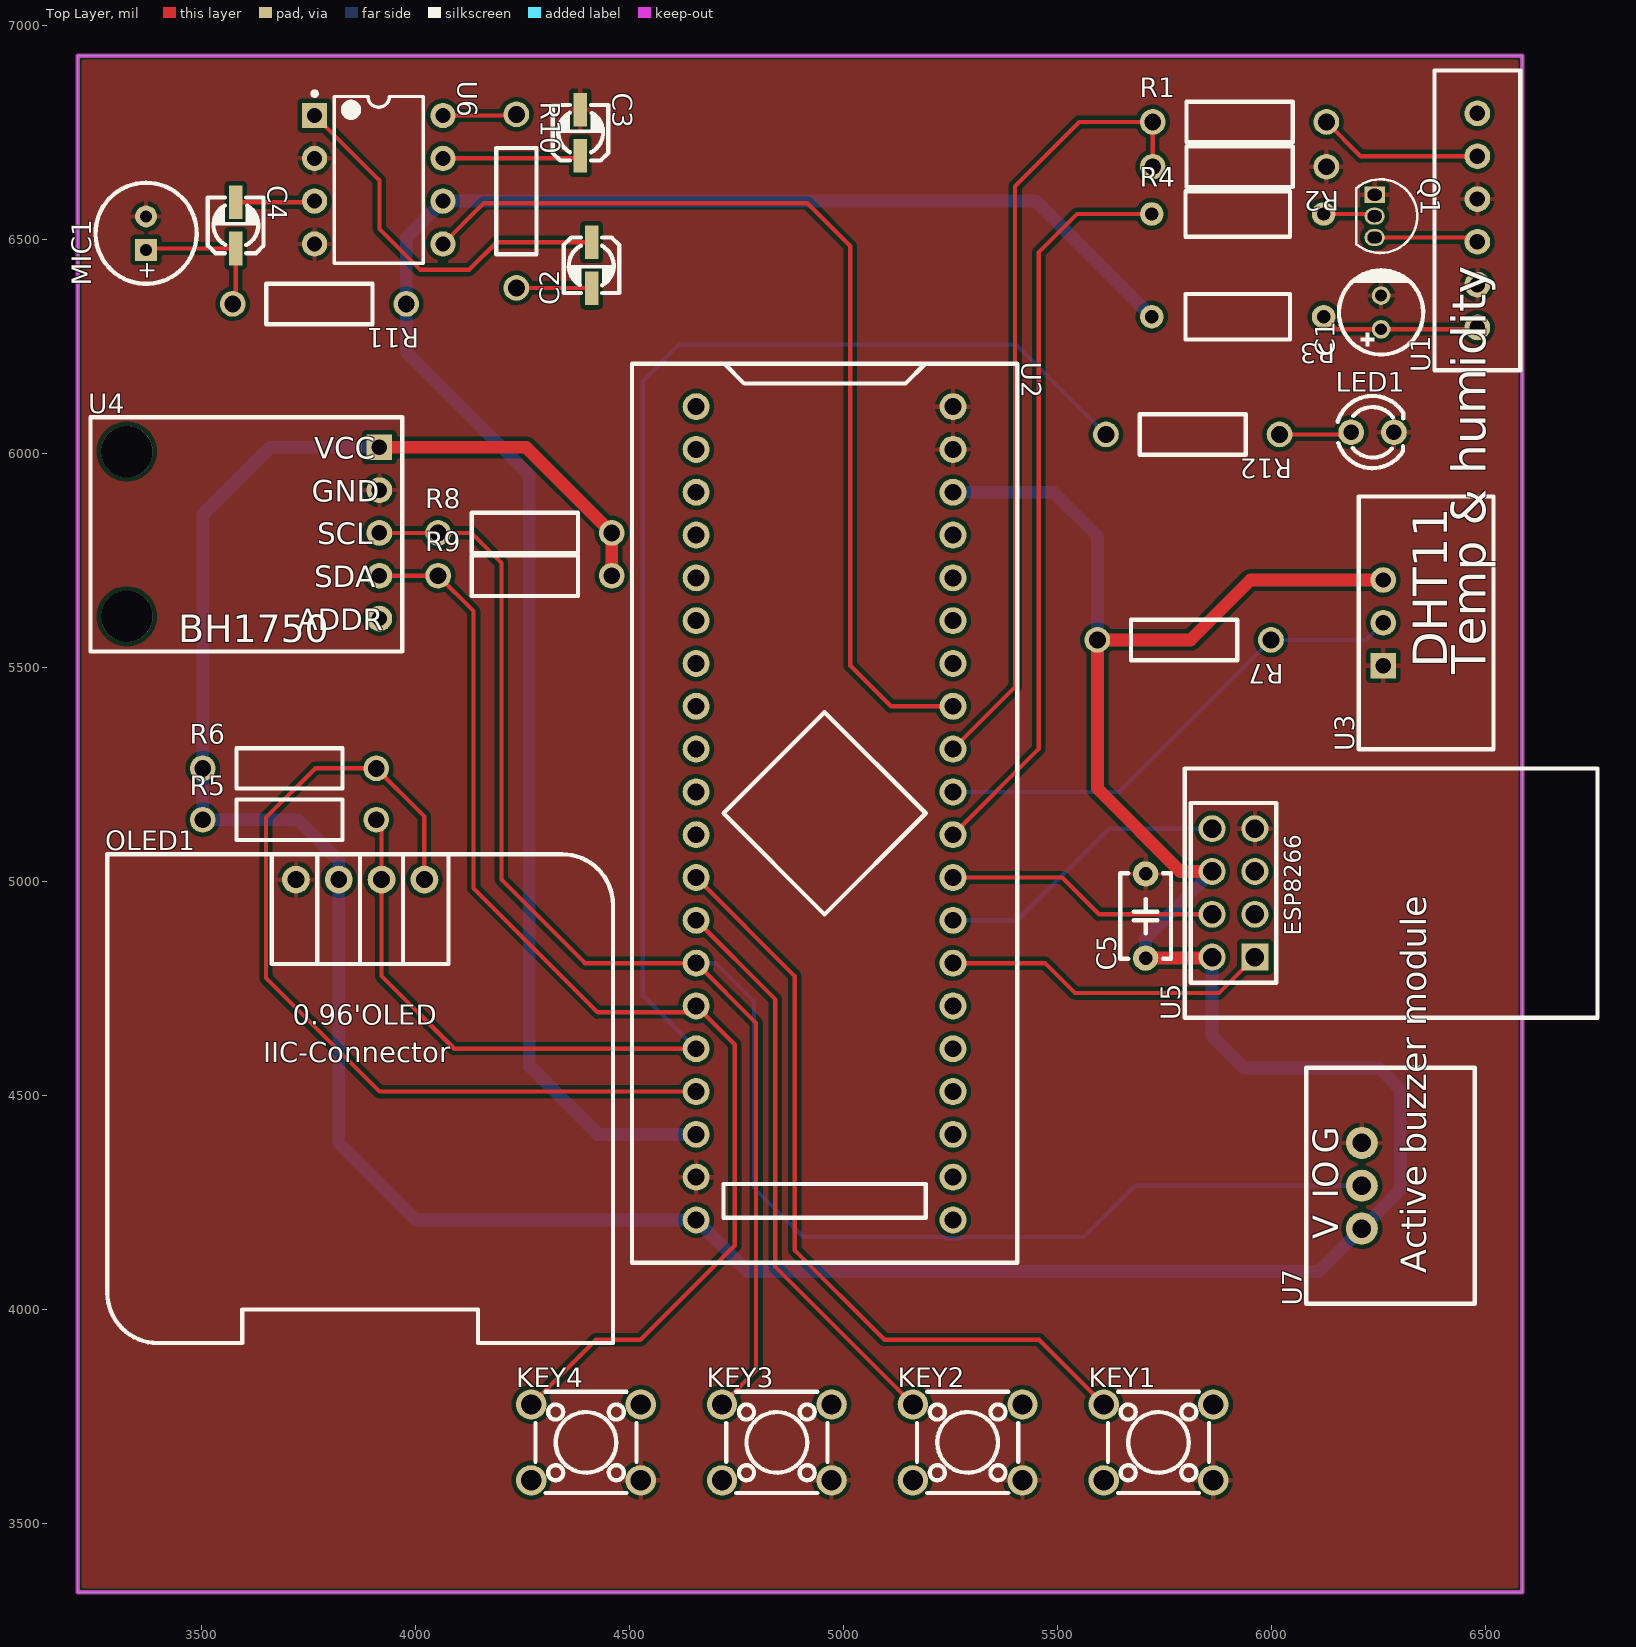
[diagram p0: Top Layer view]
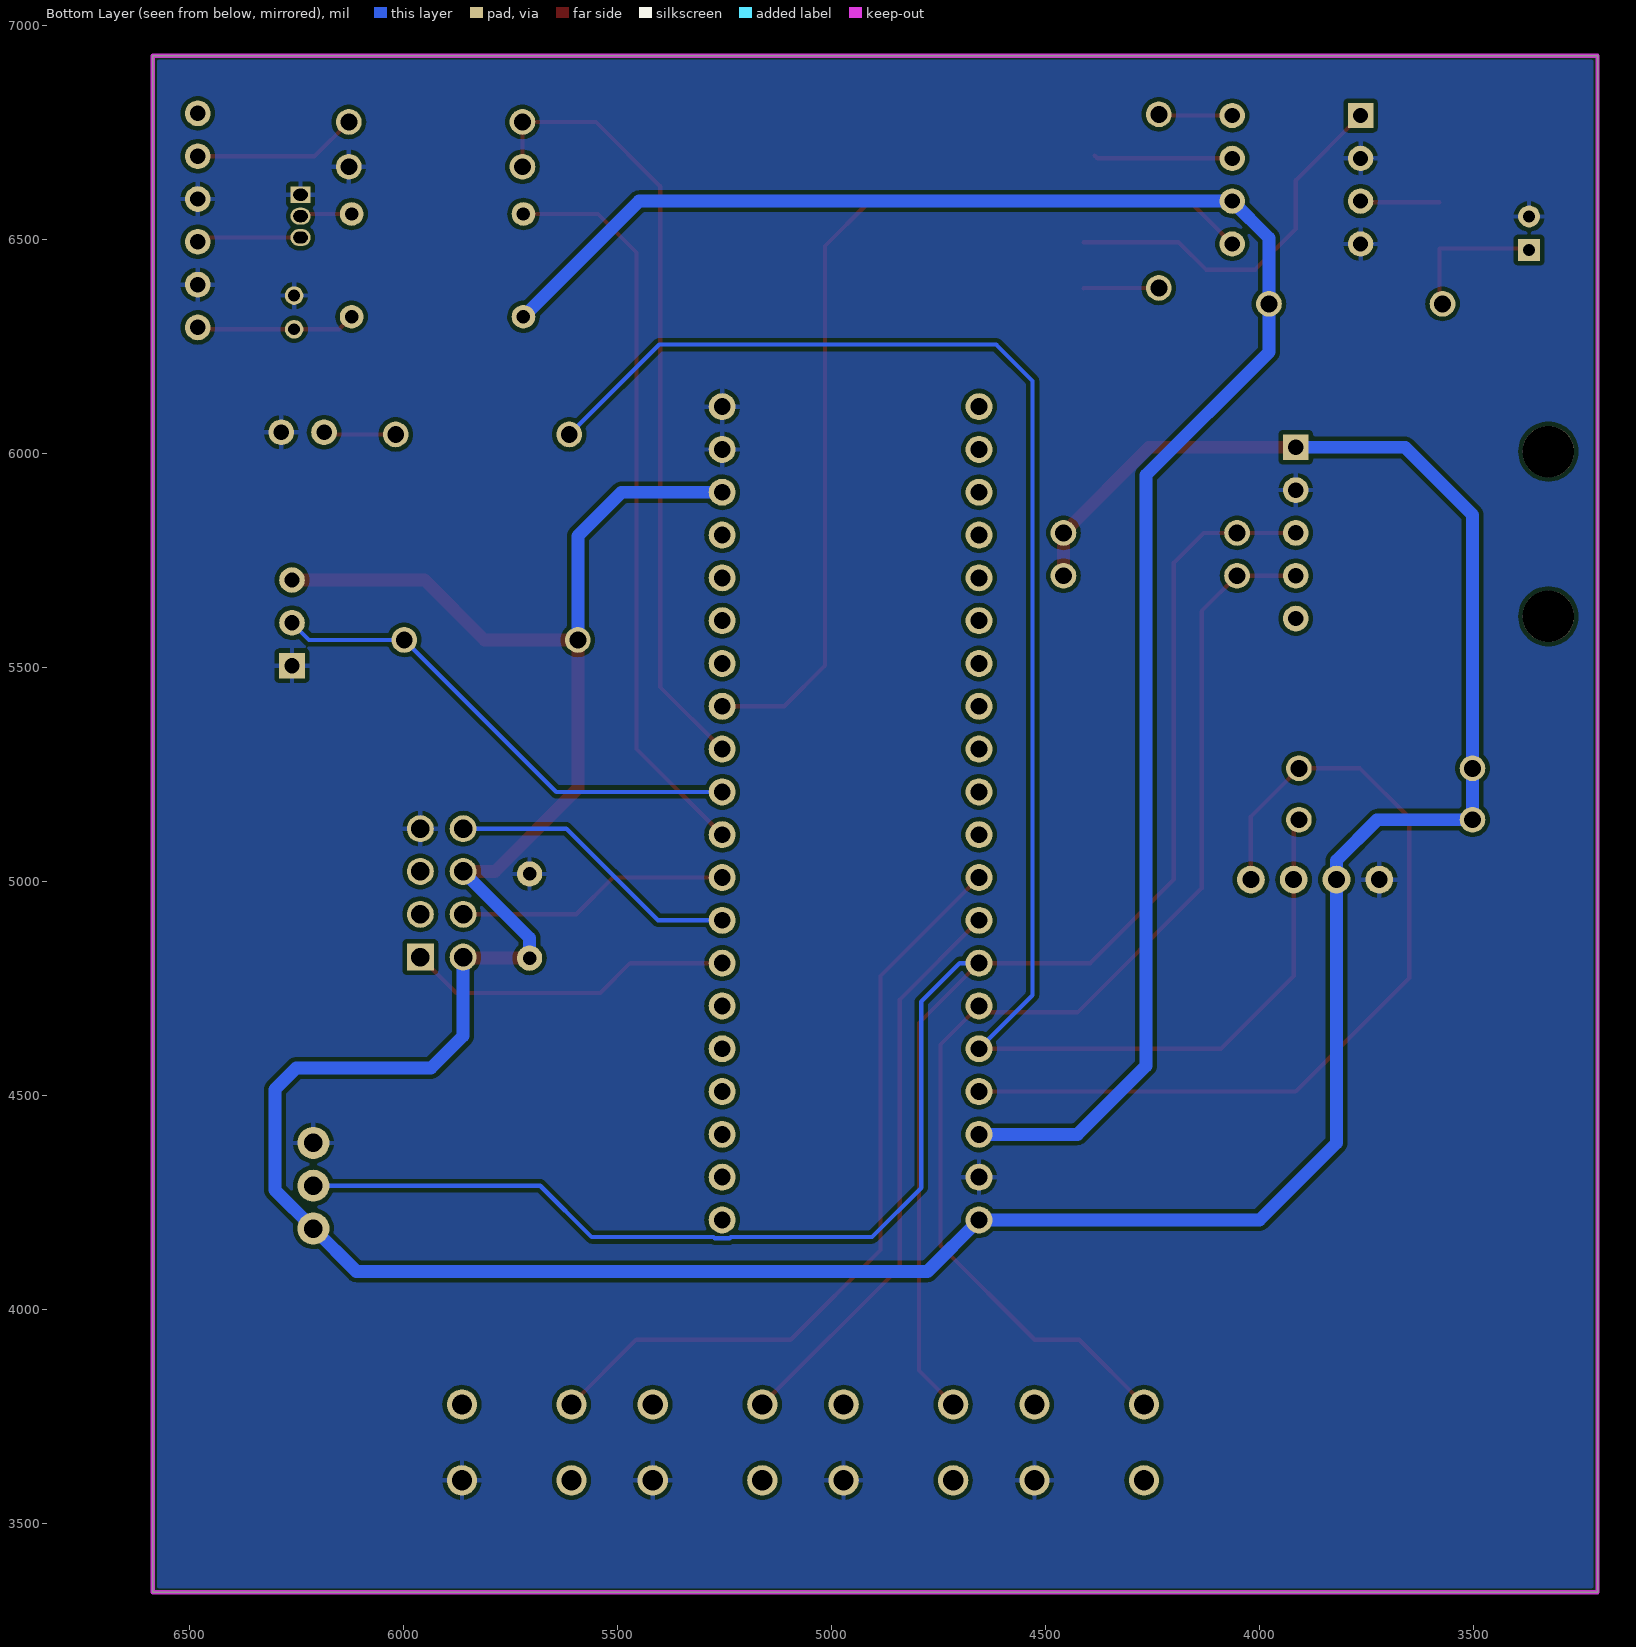
[diagram p1: Bottom Layer view, seen from below]
# Altium PCB MISC52092.pcbdoc
Units mil, origin at the board's own origin, x right, y up, seen from the top; angles counter-clockwise.
Board outline 3375 x 3590 mil, 2 copper layers (Top Layer, Bottom Layer), stack 62.206 mil thick; 32 components, 48 nets, 136 pads, 0 vias.

## Layer stack, top to bottom
Top Solder Mask Layer: solder mask 0.394, Dk 3.3
Top Layer: signal copper 1.379
Dielectric1: surface 59.449, FR4, Dk 4.5
Bottom Layer: signal copper 1.378
Bottom Solder Mask Layer: solder mask 0.394, Dk 3.3

## Board outline
3210,6930 3210,3340 6585,3340 6585,6930

## Design rules (kind name [scope] priority, off if disabled: settings)
BoardOutlineClearance copperThickness2oz_1 [All] p2 off: genericclearance=7.99 ignorepadtopadclearanceinfootprint=FALSE except(0: Arc-SplitContinuation Track-SplitContinuation SMDPad-SplitContinuation THPad-SplitContinuation Via-SplitContinuation Fill-SplitContinuation Region-SplitContinuation Poly-SplitContinuation Text-SplitContinuation Hole-SplitContinuation; 5.98: Arc-CutoutEdge SMDPad-CutoutEdge THPad-CutoutEdge Via-CutoutEdge Fill-CutoutEdge Region-CutoutEdge Text-CutoutEdge; 6.93: Hole-OutlineEdge Hole-CutoutEdge; 10: Poly-OutlineEdge Poly-CutoutEdge; 11.81: Arc-OutlineEdge Track-OutlineEdge SMDPad-OutlineEdge THPad-OutlineEdge Via-OutlineEdge Fill-OutlineEdge Region-OutlineEdge Text-OutlineEdge Track-CutoutEdge)
BoardOutlineClearance copperThickness1oz_1 [All] p4: genericclearance=4.02 ignorepadtopadclearanceinfootprint=FALSE except(0: Arc-SplitContinuation Track-SplitContinuation SMDPad-SplitContinuation THPad-SplitContinuation Via-SplitContinuation Fill-SplitContinuation Region-SplitContinuation Poly-SplitContinuation Text-SplitContinuation Hole-SplitContinuation; 6: SMDPad-CutoutEdge THPad-CutoutEdge Via-CutoutEdge Fill-CutoutEdge Region-CutoutEdge Text-CutoutEdge; 6.93: Hole-OutlineEdge Hole-CutoutEdge; 10: Poly-OutlineEdge Poly-CutoutEdge; 11.8: Arc-OutlineEdge Track-OutlineEdge SMDPad-OutlineEdge THPad-OutlineEdge Via-OutlineEdge Fill-OutlineEdge Region-OutlineEdge Text-OutlineEdge; 11.81: Arc-CutoutEdge Track-CutoutEdge)
Clearance copperThickness2oz [All] p1 off: gap=7.99 ignorepadtopadclearanceinfootprint=FALSE except(5.98: SMDPad-Track SMDPad-SMDPad THPad-Track SMDPad-THPad THPad-THPad Track-Via SMDPad-Via THPad-Via Via-Via Fill-Track Region-Track Fill-SMDPad Region-SMDPad Fill-THPad Region-THPad Fill-Via Region-Via Fill-Fill Fill-Region Region-Region Arc-Track Arc-SMDPad Arc-THPad Arc-Via Fill-Arc Region-Arc Arc-Arc Text-Track SMDPad-Text Text-THPad Text-Via Fill-Text Region-Text Arc-Text Text-Text; 6.93: Hole-Track Hole-SMDPad Hole-THPad Hole-Via Fill-Hole Region-Hole Hole-Arc Hole-Text; 10: Poly-Track Poly-SMDPad Poly-THPad Poly-Via Poly-Fill Poly-Region Poly-Poly Poly-Arc Poly-Text Poly-Hole)
Clearance copperThickness1oz [All] p3: gap=4.02 ignorepadtopadclearanceinfootprint=FALSE except(5.98: SMDPad-Track SMDPad-SMDPad THPad-Track SMDPad-THPad THPad-THPad Track-Via SMDPad-Via THPad-Via Via-Via Fill-Track Region-Track Fill-SMDPad Region-SMDPad Fill-THPad Region-THPad Fill-Via Region-Via Fill-Fill Fill-Region Region-Region; 6: Arc-Track Arc-SMDPad Arc-THPad Arc-Via Fill-Arc Region-Arc Arc-Arc Text-Track SMDPad-Text Text-THPad Text-Via Fill-Text Region-Text Arc-Text Text-Text; 6.93: Hole-Track Hole-SMDPad Hole-THPad Hole-Via Fill-Hole Region-Hole Hole-Arc Hole-Text; 10: Poly-Track Poly-SMDPad Poly-THPad Poly-Via Poly-Fill Poly-Region Poly-Poly Poly-Arc Poly-Text Poly-Hole)
DiffPairsRouting differentialPair [All] p1: maxlimit=6 minlimit=6 mostfreqgap=6 toplayer_minwidth=5 toplayer_prefwidth=10 toplayer_maxwidth=100 toplayer_mingap=6 toplayer_prefgap=6 toplayer_maxgap=6 bottomlayer_minwidth=5 bottomlayer_prefwidth=10 bottomlayer_maxwidth=100 bottomlayer_mingap=6 bottomlayer_prefgap=6 bottomlayer_maxgap=6 maxuncoupledlength=10
HoleToHoleClearance otherClearance [All] p1: gap=11.81 allowstackedmicrovias=TRUE
Length netLength [All] p1: minlimit=0 maxlimit=0
MatchedLengths netLengthTolerance [All] p1: tolerance=1000
PasteMaskExpansion pasteMaskExpansion [All] p1: expansion=0
PlaneConnect innerPlane [All] p1: planeconnectstyle=Relief reliefexpansion=20 reliefentries=4 reliefconductorwidth=10 reliefairgap=10
PolygonConnect copperRegion [(InNet('GND'))] p1: connectstyle=Relief reliefconductorwidth=10 reliefentries=4 polygonreliefangle="90 Angle" airgapwidth=10 via.connectstyle=Relief via.reliefconductorwidth=10 via.reliefentries=4 via.polygonreliefangle="90 Angle" via.airgapwidth=10
RoutingVias viaSize [All] p1: holewidth=12.01 width=24.02 viastyle="Through Hole" minholewidth=11.81 minwidth=19.68 maxholewidth=248.03 maxwidth=393.7
SolderMaskExpansion solderMaskExpansion [IsVia] p1: expansion=-1000 istentingtop=TRUE
SolderMaskExpansion solderMaskExpansion [All] p2: expansion=2 istentingtop=FALSE
Width copperThickness2oz_2 [All] p1 off: maxlimit=100 minlimit=8 preferedwidth=10
Width copperThickness1oz_2 [All] p2: maxlimit=100 minlimit=5 preferedwidth=10

## Components (designator, comment, footprint, x,y, rotation, side; value= is the part's Value field where it differs from the comment)
C1 "10uF" CAP-TH_BD5.0-P2.00-D0.5-FD 6255,6330 r90 top
C2 "10uF" C_Ele_SMD_3x5.4mm 4410,6440 r90 top
C3 "10uF" C_Ele_SMD_3x5.4mm 4385,6750 r270 top
C4 "10uF" C_Ele_SMD_3x5.4mm 3579.65,6533.55 r270 top
C5 "5pF" CAP-TH_L5.0-W3.0-P5.00-D0.6 5705,4920 r90 top
KEY1 "" SW-TH_4P-L6.0-W6.0-P4.50-LS6.5 5735,3690.4 r0 top
KEY2 "" SW-TH_4P-L6.0-W6.0-P4.50-LS6.5 5289.21,3690.4 r0 top
KEY3 "" SW-TH_4P-L6.0-W6.0-P4.50-LS6.5 4843.42,3690.4 r0 top
KEY4 "" SW-TH_4P-L6.0-W6.0-P4.50-LS6.5 4397.63,3690.4 r0 top
LED1 "" LED_TH-3mm 6235,6050 r0 top
MIC1 "MIC" MIC-TH_BD6.0-P2.00 3370,6515 r90 top
OLED1 "0.96OLED_4P_MODULE_JX" 0.96OLED_4P 3870,5005 r0 top
Q1 "S8050" TO-92-3_L4.5-W3.5-P1.27-L 6240,6555 r270 top
R1 "10kΩ" Res_1/4W 5924.41,6775 r0 top
R2 "10kΩ" Res_1/4W 5924.41,6670.45 r180 top
R3 "10kΩ" RES-TH_BD2.7-L6.2-P10.20-D0.4 5920,6320 r180 top
R4 "1kΩ" RES-TH_BD2.7-L6.2-P10.20-D0.4 5920,6560 r0 top
R5 "10kΩ" Res_1/4W 3705,5145 r0 top
R6 "10kΩ" Res_1/4W 3705,5265 r0 top
R7 "4.7K" Res_1/4W 5795,5565 r180 top
R8 "10kΩ" Res_1/4W 4255,5815 r0 top
R9 "10kΩ" Res_1/4W 4255,5715 r0 top
R10 "3kΩ" Res_1/4W 4235,6590 r270 top
R11 "100kΩ" Res_1/4W 3775,6350 r180 top
R12 "10kΩ" Res_1/4W 5815,6045 r180 top
U1 "PM2.5 sensor_GP2Y1014AU" PM2.5传感器_GP2Y1014AU 6480,6295 r90 top
U2 "STM32F103C8T6-Card" CONN-TH_L53.3-W22.9_STM32F103C8T6-CARD 4955,5160 r270 top
U3 "DHT11" DHT11 6460,5505 r90 top
U4 "" BH1750光照传感器 3655,5805 r0 top
U5 "" ESP8266-1 5910.21,4974.09 r90 top
U6 "LM386N-3/NOPB" DIP-8_L9.8-W6.6-P2.54-LS7.6-BL 3913.53,6640 r270 top
U7 "" 有源蜂鸣器模块 6210,4190 r90 top

## Footprints (in the part's own frame and the unit in brackets; to place one, negate y for a bottom-side part, rotate by r counter-clockwise, add the part's x,y. Pads: shape width x height; smd on the part's side, far side on the other; paste and mask are expansions set on the pad)
0.96OLED_4P [mm]
  round 1.65 hole 1 copper offset 0,0: 1(-3.81,-0.001) 2(-1.27,0.002) 3(1.27,0.002) 4(3.81,0.002)
  silkscreen extent -15,-27.5 15,1.5
BH1750光照传感器 [mil]
  rect 60x60 hole 36: 1(260,210)
  round 60 hole 36: 2(260,110) 3(260,10) 4(260,-90) 5(260,-190)
  round 120 hole 120 unplated: ""(-330,-185) ""(-330,200)
  silkscreen extent -415,-267 313,280
C_Ele_SMD_3x5.4mm [mil]
  rect 78.7x31.5 smd paste+0 mask+2: 1(54.1,-0.55) 2(-53.7,-0.55)
  silkscreen extent -65,-65 65,65
CAP-TH_BD5.0-P2.00-D0.5-FD [mm]
  round 1.1 hole 0.7 paste+0 mask+0.05: 1(-1,0) 2(1,0)
  silkscreen extent -2.5,-2.5 2.5,2.5
CAP-TH_L5.0-W3.0-P5.00-D0.6 [mm]
  round 1.5 hole 0.8: 1(-2.5,0) 2(2.5,0)
  silkscreen extent -2.54,-1.5 2.54,1.5
CONN-TH_L53.3-W22.9_STM32F103C8T6-CARD [mm]
  round 1.6 hole 1: 1(-24.13,-7.62) 2(-21.59,-7.62) 3(-19.05,-7.62) 4(-16.51,-7.62) 5(-13.97,-7.62) 6(-11.43,-7.62) 7(-8.89,-7.62) 8(-6.35,-7.62) 9(-3.81,-7.62) 10(-1.27,-7.62) 11(1.27,-7.62) 12(3.81,-7.62) 13(6.35,-7.62) 14(8.89,-7.62) 15(11.43,-7.62) 16(13.97,-7.62) 17(16.51,-7.62) 18(19.05,-7.62) 19(21.59,-7.62) 20(24.13,-7.62) 21(24.13,7.62) 22(21.59,7.62) 23(19.05,7.62) 24(16.51,7.62) 25(13.97,7.62) 26(11.43,7.62) 27(8.89,7.62) 28(6.35,7.62) 29(3.81,7.62) 30(1.27,7.62) 31(-1.27,7.62) 32(-3.81,7.62) 33(-6.35,7.62) 34(-8.89,7.62) 35(-11.43,7.62) 36(-13.97,7.62) 37(-16.51,7.62) 38(-19.05,7.62) 39(-21.59,7.62) 40(-24.13,7.62)
  silkscreen extent -26.67,-11.43 26.67,11.43
DHT11 [mil]
  rect 60x60 hole 36 paste+0 mask+4: 1(-0.01,200.01)
  round 60 hole 36 paste+0 mask+2: 2(99.99,200.01)
  round 60 hole 36 paste+0 mask+4: 3(199.99,200.01)
  silkscreen extent -195,-57 395,257
DIP-8_L9.8-W6.6-P2.54-LS7.6-BL [mm]
  rect 1.5x1.5 hole 0.9: 1(-3.81,-3.81)
  round 1.5 hole 0.9: 2(-1.27,-3.81) 3(1.27,-3.81) 4(3.81,-3.81) 5(3.81,3.81) 6(1.27,3.81) 7(-1.27,3.81) 8(-3.81,3.81)
  silkscreen extent -5.23,-3.93 4.96,2.65
ESP8266-1 [mm]
  rect 1.6x1.6 hole 1.1: 1(-3.81,-1.27)
  round 1.6 hole 1.1: 2(-3.81,1.27) 3(-1.27,-1.27) 4(-1.27,1.27) 5(1.27,-1.27) 6(1.27,1.27) 7(3.81,-1.27) 8(3.81,1.27)
  silkscreen extent -7.42,-21.6 7.38,2.9
LED_TH-3mm [mil]
  round 60 hole 36 paste+0 mask+2: 1(-50,0) 2(50,0)
  silkscreen extent -81,-84 72,85
MIC-TH_BD6.0-P2.00 [mm]
  rect 1.3x1.3 hole 0.7: 1(-1,0)
  round 1.3 hole 0.7: 2(1,0)
  silkscreen extent -3,-3 3,3
PM2.5传感器_GP2Y1014AU [mil]
  round 60 hole 36 paste+0 mask+4: 1(0,0) 2(100,0) 3(200,0) 4(300,0) 5(400,0) 6(500,0)
  silkscreen extent -100,-100 600,100
RES-TH_BD2.7-L6.2-P10.20-D0.4 [mm]
  round 1.4 hole 0.8 copper offset 0,0: 1(-5.1,0) 2(5.1,0)
  silkscreen extent -3.1,-1.35 3.1,1.35
Res_1/4W [mil]
  round 60 hole 39.37 paste+0 mask+2: 1(-202.76,0) 2(202.76,0)
  silkscreen extent -124,-47 124,47
SW-TH_4P-L6.0-W6.0-P4.50-LS6.5 [mm]
  round 1.8 hole 1.2: 1(-3.25,2.25) 2(3.25,2.25) 3(-3.25,-2.25) 4(3.25,-2.25)
  silkscreen extent -3,-3 3,3
TO-92-3_L4.5-W3.5-P1.27-L [mm]
  rect 1x1.2 hole 0.7 slot 0.85 at 90 deg: 1(-1.27,0)
  oval 1x1.2 hole 0.7 slot 0.85 at 90 deg: 2(0,0) 3(1.27,0)
  silkscreen extent -2.19,-1.1 2.19,2.52
有源蜂鸣器模块 [mil]
  round 74.8 hole 43.31: 1(0,0) 2(100,0) 3(200,0)
  silkscreen extent -176,-264 376,130

## Nets (pads, with @x,y where several pads share a name; then routed paths per layer and width w, separated by ;. In a path a pad name is that pad's centre, name@x,y a point inside that pad or via, vN(x,y) a via of type N, cw(c..) or ccw(c..) an arc to the next point about the centre after c; other vN are vias at no path point)
3.3V: C5.1 OLED1.2 R5.1 R6.1 R7.2 R8.2 R9.2 U2.20 U2.38 U3.3 U4.1 U5.2 U5.6 U7.1 | length 8993.4
  Top Layer w30: U4.1 4257.76,6015 R8.2 R9.2 ; C5.1 5857.7,4821.57 U5.2 ; U5.6 5785.91,5024.09 5592.24,5217.76 R7.2 5810,5565 5949.99,5704.99 U3.3
  Bottom Layer w30: U4.1 3660,6015 3502.24,5857.24 R6.1 R5.1 3725,5145 3820,5050 3820,5005.05 3820,4390 4000,4210 U2.20 4775,4090 6110,4090 U7.1 6300,4280 6300,4515 6250,4565 5935,4565 5860.21,4639.79 U5.2 ; U2.38 5490,5910 5592.24,5807.76 R7.2 ; C5.1 5705,4868.87 U5.6
5V: R3.2 R11.1 U2.18 U6.6 | length 4398.3
  Bottom Layer w30: U2.18 4425,4410 4265,4570 4265,5950 3977.76,6237.24 R11.1 3977.76,6504.23 U6.6 5449.21,6590 R3.2
$1N5: Q1.2 R4.2 | length 121.3
  Top Layer w10: R4.2 6235,6560 Q1.2
$1N6: Q1.3 U1.3 | length 244.1
  Top Layer w10: Q1.3 6470,6505 U1.3
$1N9: R1.2 U1.5 | length 386
  Top Layer w10: R1.2 6207.17,6695 U1.5
$1N11: C1.1 R3.1 U1.1 | length 373.2
  Top Layer w10: R3.1 6150.16,6290.63 C1.1 6475.63,6290.63 U1.1
$1N62: C2.1 U6.1 | length 889.2
  Top Layer w10: U6.1 3915,6638.53 3915,6525 4010,6430 4125,6430 4189.1,6494.1 C2.1
$1N63: C2.2 R10.2 | length 175.9
  Top Layer w10: R10.2 4409.61,6387.24 C2.2
$1N64: R10.1 U6.8 | length 172.6
  Top Layer w10: U6.8 4232.24,6790 R10.1
$1N65: C3.1 U6.7 | length 323.4
  Top Layer w10: U6.7 4378.55,6690 C3.1
$1N67: C4.2 U6.3 | length 185.6
  Top Layer w10: C4.2 3760.78,6587.25 U6.3
$1N70: C4.1 MIC1.1 R11.2 | length 343
  Top Layer w10: MIC1.1 3373.82,6479.45 C4.1 3579.1,6356.86 R11.2
$1N80: LED1.1 R12.1 | length 169.3
  Top Layer w10: R12.1 6180,6045 LED1.1
+5V: U1.6
GND: C1.2 C3.2 C5.2 KEY1.4 KEY2.4 KEY3.4 KEY4.4 LED1.2 MIC1.2 OLED1.1 Q1.1 R2.1 U1.2 U1.4 U2.19 U2.39 U2.40 U3.1 U4.2 U5.7 U6.2 U6.4 U7.3
NRST: U2.37
PA0: U2.25
PA1: U2.26
PA2: U2.27 U5.1 | length 769
  Top Layer w10: U2.27 5470,4810 5540,4740 5876.13,4740 U5.1
PA3: U2.28 U5.8 | length 693.9
  Bottom Layer w10: U2.28 5405,4910 5619.09,5124.09 U5.8
PA4: U2.29 U5.4 | length 640.8
  Top Layer w10: U2.29 5510,5010 5595.91,4924.09 U5.4
PA5: R4.1 U2.30 | length 1744.3
  Top Layer w10: U2.30 5455,5310 5455,6470 5545,6560 R4.1
PA6: R7.1 U2.31 U3.2 | length 1168.6
  Bottom Layer w10: U2.31 5642.76,5210 R7.1 6220,5565 U3.2
PA7: R1.1 R2.2 U2.32 | length 1863.4
  Top Layer w10: U2.32 5400,5455 5400,6625 5550,6775 R1.1 R2.2
PA8: U2.5
PA9: U2.6
PA10: U2.7
PA11: U2.8
PA12: U2.9
PA15: U2.10
PB0: U2.33 U6.5 | length 2291.6
  Top Layer w10: U6.5 4158.53,6585 4915,6585 5015,6485 5015,5505 5110,5410 U2.33
PB1: U2.34
PB3: U2.11
PB4: KEY1.1 U2.12 | length 1836.9
  Top Layer w10: U2.12 4885,4780 4885,4140 5095,3930 5456.03,3930 KEY1.1
PB5: KEY2.1 U2.13 | length 1340.7
  Top Layer w10: U2.13 4840,4725 4840,4100.24 KEY2.1
PB6: KEY3.1 R8.1 U2.14 U4.3 U7.2 | length 4838.4
  Top Layer w10: U4.3 R8.1 4130,5815 4200,5745 4200,5005 4395,4810 U2.14 4795,4670 4795,3858.52 KEY3.1
  Bottom Layer w10: U2.14 4700,4810 4790,4720 4790,4285 4905,4170 5234.92,4170 5237.41,4167.52 5272.6,4167.52 5275.08,4170 5560,4170 5680,4290 U7.2
PB7: KEY4.1 R9.1 U2.15 U4.4 | length 2774.1
  Top Layer w10: U4.4 R9.1 4135,5632.24 4135,4985 4425,4695 4640,4695 U2.15 4745,4620 4745,4150 4525,3930 4420.69,3930 KEY4.1
PB8: OLED1.3 R5.2 R12.2 U2.16 | length 3991.7
  Top Layer w10: R5.2 3920,5132.76 3920,5005.05 3920,4780 4090,4610 U2.16
  Bottom Layer w10: U2.16 4530,4735 4530,6170 4615,6255 5402.24,6255 R12.2
PB9: OLED1.4 R6.2 U2.17 | length 2101.6
  Top Layer w10: OLED1.4@4020,5005.05 4020,5152.76 R6.2 3765,5265 3650,5150 3650,4775 3915,4510 U2.17
PB10: U2.35
PB11: U2.36
PB12: U2.1
PB13: U2.2
PB14: U2.3
PB15: U2.4
PC13: U2.22
PC14: U2.23
PC15: U2.24
pads on no net: KEY1.2 KEY1.3 KEY2.2 KEY2.3 KEY3.2 KEY3.3 KEY4.2 KEY4.3 U2.21 U4. U4.5 U5.3 U5.5

## Polygon pours and split planes (outlines as drawn)
GND on Top Layer (solid, remove dead copper, pour order 0): 3000,7060 3000,3000 7245,3000 7245,7060
GND on Bottom Layer (solid, remove dead copper, pour order 2): 3020,7175 3020,3035 6800,3035 6800,7175

## Keep-outs
Board Outline Layer:
  the board outline again, w10